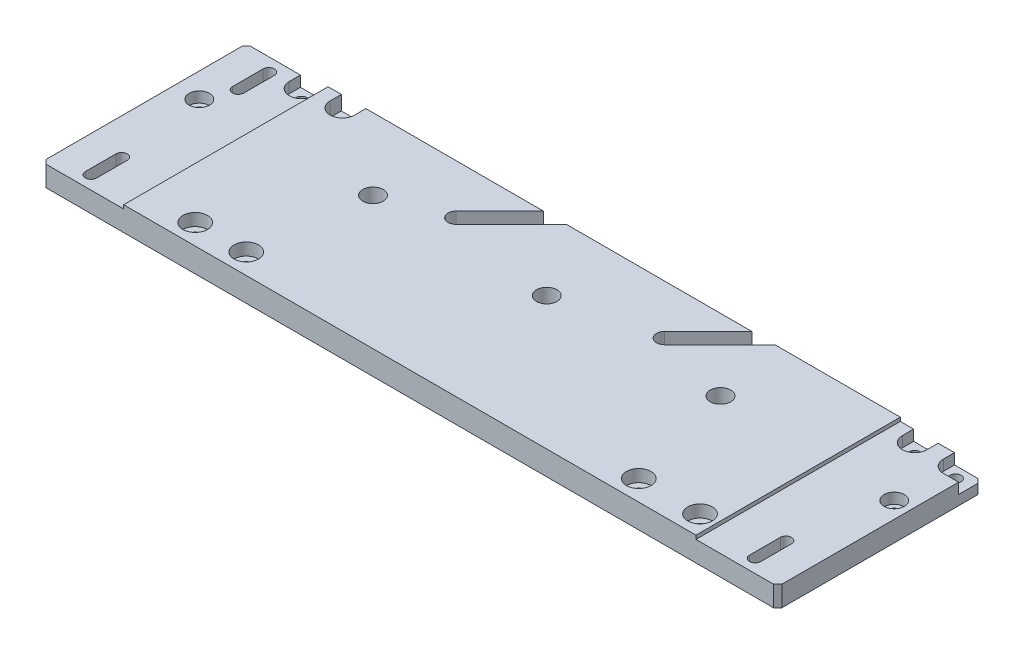
SolidWorks part; units mm, degrees
ref_plane "Front Plane" through (0, 0, 0) normal (0, 0, 1) x (1, 0, 0)
ref_plane "Top Plane" through (0, 0, 0) normal (0, 1, 0) x (1, 0, 0)
ref_plane "Right Plane" through (0, 0, 0) normal (1, 0, 0) x (0, 0, -1)
sketch "Sketch1" plane through (0, 0, 0) normal (0, 1, 0) x (1, 0, 0)
  line L1 (-180, 50) -> (180, 50)
  line L2 (-180, 50) -> (-180, -50)
  line L3 (-180, -50) -> (180, -50)
  line L4 (180, 50) -> (180, -50)
  line L5 (-180, 50) -> (180, -50) construction
  line L6 (-180, -50) -> (180, 50) construction
  point P0 (0, 0)
  dimension "D1" = 360
  dimension "D2" = 100
extrude "Boss-Extrude1" add sketch "Sketch1" along normal blind 10
sketch "Sketch2" plane through (0, 10, 0) normal (0, 1, 0) x (1, 0, 0)
  line L0 (180, 50) -> (-180, 50) construction
  line L1 (-140, -50) -> (140, -50)
  line L2 (-140, -50) -> (-140, 50)
  line L3 (-140, 50) -> (140, 50)
  line L4 (140, -50) -> (140, 50)
  line L5 (-140, -50) -> (140, 50) construction
  line L6 (-140, 50) -> (140, -50) construction
  point P0 (0, 0)
  dimension "D1" = 280
extrude "Boss-Extrude2" add sketch "Sketch2" along normal blind 1.8
sketch "Sketch3" plane through (0, 0, 0) normal (0, -1, 0) x (1, 0, 0)
  line L0 (-32.2377, -40) -> (49967.7623, -40) construction
  line L2 (-180, -50) -> (-180, 50) construction
  line L3 (180, -50) -> (-180, -50) construction
  circle A0 centre (-39, -40) radius 4
  circle A1 centre (63, -40) radius 4
  dimension "D1" = 102
  dimension "D3" = 8
  dimension "D4" = 141
  dimension "D2" = 10
extrude "Cut-Extrude1" cut sketch "Sketch3" against normal through all
sketch "Sketch4" plane through (0, 0, 0) normal (0, -1, 0) x (1, 0, 0)
  line L0 (-56.0102, -57.0102) -> (35299.3289, 35298.3289) construction
  line L1 (53.9844, -49.0156) -> (35409.3234, 35306.3234) construction
  line L3 (180, -50) -> (-180, -50) construction
  line L4 (-64.5, -14.5) -> (35290.8391, -35369.8391) construction
  line L5 (44, -21) -> (35399.3391, -35376.3391) construction
  line L6 (48.8579, -25.8579) -> (77.1421, -54.1421) construction
  line L7 (51.6863, -23.0294) -> (79.9706, -51.3137)
  line L8 (46.0294, -28.6863) -> (74.3137, -56.9706)
  line L9 (-53.1421, -25.8579) -> (-24.8579, -54.1421) construction
  line L10 (-50.3137, -23.0294) -> (-22.0294, -51.3137)
  line L11 (-55.9706, -28.6863) -> (-27.6863, -56.9706)
  arc A0 (51.6863, -23.0294) -> (46.0294, -28.6863) centre (48.8579, -25.8579) ccw
  arc A1 (74.3137, -56.9706) -> (79.9706, -51.3137) centre (77.1421, -54.1421) ccw
  arc A2 (-50.3137, -23.0294) -> (-55.9706, -28.6863) centre (-53.1421, -25.8579) ccw
  arc A3 (-27.6863, -56.9706) -> (-22.0294, -51.3137) centre (-24.8579, -54.1421) ccw
  circle A4 centre (-39, -40) radius 4 construction
  point P14 (63, -40)
  point P20 (-39, -40)
  dimension "D1" = 45
  dimension "D2" = 40
  dimension "D3" = 40
extrude "Cut-Extrude2" cut sketch "Sketch4" against normal blind 39
sketch "Sketch5" plane through (0, 0, 0) normal (0, -1, 0) x (1, 0, 0)
  line L0 (-160, 0) -> (49840, 0) construction
  line L1 (-180, -50) -> (-180, 50) construction
  line L2 (-162.504, 43.5) -> (-162.496, 28.5) construction
  line L3 (-159.754, 43.5015) -> (-159.746, 28.5015)
  line L4 (-165.254, 43.4985) -> (-165.246, 28.4985)
  line L6 (0, 50) -> (0, -49950) construction
  line L7 (-180, 50) -> (180, 50) construction
  line L8 (162.5, 43.5) -> (162.5, 28.5) construction
  line L9 (159.75, 43.5) -> (159.75, 28.5)
  line L10 (165.25, 43.5) -> (165.25, 28.5)
  line L23 (-162.504, -43.5) -> (-162.496, -28.5) construction
  line L24 (-159.754, -43.5015) -> (-159.746, -28.5015)
  line L25 (-165.254, -43.4985) -> (-165.246, -28.4985)
  arc A0 (-159.754, 43.5015) -> (-165.254, 43.4985) centre (-162.504, 43.5) ccw
  arc A1 (-165.246, 28.4985) -> (-159.746, 28.5015) centre (-162.496, 28.5) ccw
  arc A2 (159.75, 43.5) -> (165.25, 43.5) centre (162.5, 43.5) cw
  arc A3 (165.25, 28.5) -> (159.75, 28.5) centre (162.5, 28.5) cw
  arc A12 (-159.754, -43.5015) -> (-165.254, -43.4985) centre (-162.504, -43.5) cw
  arc A13 (-165.246, -28.4985) -> (-159.746, -28.5015) centre (-162.496, -28.5) cw
  point P4 (-180, 0)
  point P7 (-162.5, 36)
  point P18 (0, 50)
  point P19 (162.5, 36)
  point P55 (-162.5, -36)
  dimension "D1" = 5.5
  dimension "D2" = 15
  dimension "D3" = 325
  dimension "D4" = 72
  dimension "D5" = 5.5
  dimension "D6" = 15
extrude "Cut-Extrude3" cut sketch "Sketch5" against normal blind 39
chamfer "Chamfer1" distance 2 angle 45 6 edges at (180, 5, 50) (-180, 5, 50) (-180, 5, -50) (180, 5, -50)
sketch "Sketch6" plane through (0, 11.8, 0) normal (0, 1, 0) x (1, 0, 0)
  line L0 (180, -48) -> (180, 48) construction
  line L1 (-140, -50) -> (140, -50) construction
  circle A0 centre (132, -40) radius 2.75
  circle A1 centre (102, -40) radius 2.75
  circle A2 centre (-90, -40) radius 2.75
  circle A3 centre (-115, -40) radius 2.75
  dimension "D6" = 5.5
  dimension "D1" = 30
  dimension "D2" = 25
  dimension "D3" = 48
  dimension "D4" = 270
  dimension "D5" = 10
extrude "Cut-Extrude4" cut sketch "Sketch6" against normal through all
sketch "Sketch7" plane through (0, 11.8, 0) normal (0, 1, 0) x (1, 0, 0)
  circle A0 centre (-115, -40) radius 6
  circle A1 centre (-90, -40) radius 6
  circle A2 centre (102, -40) radius 6
  circle A3 centre (132, -40) radius 6
  dimension "D1" = 12
extrude "Cut-Extrude5" cut sketch "Sketch7" against normal blind 6
sketch "Sketch8" plane through (0, 11.8, 0) normal (0, 1, 0) x (1, 0, 0)
  line L0 (-180, 48) -> (-180, -48) construction
  line L1 (-34.6569, 50) -> (-140, 50) construction
  circle A0 centre (-147.5, 44.5) radius 2.75
  circle A1 centre (-127.5, 44.5) radius 2.75
  dimension "D1" = 5.5
  dimension "D2" = 20
  dimension "D3" = 32.5
  dimension "D4" = 5.5
extrude "Cut-Extrude6" cut sketch "Sketch8" against normal blind 19
sketch "Sketch9" plane through (0, 11.8, 0) normal (0, 1, 0) x (1, 0, 0)
  circle A0 centre (-147.5, 44.5) radius 6
  circle A1 centre (-127.5, 44.5) radius 6
  dimension "D1" = 12
extrude "Cut-Extrude7" cut sketch "Sketch9" against normal blind 7
sketch "Sketch11" plane through (0, 11.8, 0) normal (0, 1, 0) x (1, 0, 0)
  line L0 (-147.5, 44.5) -> (-147.5, 50044.5) construction
  line L1 (-127.5, 44.5) -> (-127.5, 50044.5) construction
  line L2 (-125.1021, 50) -> (-129.8979, 50) construction
  line L3 (-153.5, 56.0023) -> (-141.5, 56.0023)
  line L4 (-153.5, 56.0023) -> (-153.5, 44.5)
  line L5 (-153.5, 44.5) -> (-141.5, 44.5)
  line L6 (-141.5, 56.0023) -> (-141.5, 44.5)
  line L7 (-153.5, 56.0023) -> (-141.5, 44.5) construction
  line L8 (-153.5, 44.5) -> (-141.5, 56.0023) construction
  line L9 (-133.5, 55.5) -> (-121.5, 55.5)
  line L10 (-133.5, 55.5) -> (-133.5, 44.5)
  line L11 (-133.5, 44.5) -> (-121.5, 44.5)
  line L12 (-121.5, 55.5) -> (-121.5, 44.5)
  line L13 (-133.5, 55.5) -> (-121.5, 44.5) construction
  line L14 (-133.5, 44.5) -> (-121.5, 55.5) construction
  arc A0 (-149.8979, 50) -> (-145.1021, 50) centre (-147.5, 44.5) ccw construction
  arc A1 (-149.8979, 50) -> (-145.1021, 50) centre (-147.5, 44.5) ccw construction
  arc A2 (-129.8979, 50) -> (-125.1021, 50) centre (-127.5, 44.5) ccw construction
  arc A3 (-129.8979, 50) -> (-125.1021, 50) centre (-127.5, 44.5) ccw construction
  point P6 (-147.5, 50.2511)
  point P17 (-127.5, 50)
extrude "Cut-Extrude8" cut sketch "Sketch11" against normal up to surface (7 mm away) up to face at (-147.5, 4.8, -41.75)
sketch "Sketch12" plane through (0, 11.8, 0) normal (0, 1, 0) x (1, 0, 0)
  line L0 (-180, 48) -> (-180, -48) construction
  line L1 (-178, -50) -> (-140, -50) construction
  circle A0 centre (-168, 15) radius 2.75
  dimension "D1" = 5.5
  dimension "D2" = 12
  dimension "D3" = 65
extrude "Cut-Extrude9" cut sketch "Sketch12" against normal through all
pattern_linear "LPattern1" count 5 spacing 85 along (1, 0, 0) of "Cut-Extrude9"
sketch "Sketch13" plane through (0, 11.8, 0) normal (0, 1, 0) x (1, 0, 0)
  circle A0 centre (172, 15) radius 5
  circle A1 centre (87, 15) radius 5
  circle A2 centre (2, 15) radius 5
  circle A3 centre (-83, 15) radius 5
  circle A4 centre (-168, 15) radius 5
  dimension "D1" = 10
extrude "Cut-Extrude10" cut sketch "Sketch13" against normal blind 7
sketch "Sketch14" plane through (0, 0, 0) normal (0, -1, 0) x (1, 0, 0)
  circle A0 centre (152.5, -44.5) radius 2.75
  circle A1 centre (172.5, -44.5) radius 2.75
  dimension "D1" = 5.5
extrude "Cut-Extrude11" cut sketch "Sketch14" against normal blind 10
sketch "Sketch15" plane through (0, 10, 0) normal (0, 1, 0) x (1, 0, 0)
  circle A0 centre (152.5, 44.5) radius 6
  circle A1 centre (172.5, 44.5) radius 6
  arc A2 (-133.5, 44.5) -> (-121.5, 44.5) centre (-127.5, 44.5) ccw construction
extrude "Cut-Extrude12" cut sketch "Sketch15" against normal up to surface (5.2 mm away)
sketch "Sketch16" plane through (0, 10, 0) normal (0, 1, 0) x (1, 0, 0)
  line L0 (152.5, 44.5) -> (50152.5, 44.5) construction
  line L1 (172.5, 44.5) -> (172.5, 50044.5) construction
  line L2 (152.5, 44.5) -> (152.5, 50044.5) construction
  line L3 (154.8979, 50) -> (150.1021, 50) construction
  line L4 (146.5, 55.5) -> (158.5, 55.5)
  line L5 (146.5, 55.5) -> (146.5, 44.5)
  line L6 (146.5, 44.5) -> (158.5, 44.5)
  line L7 (158.5, 55.5) -> (158.5, 44.5)
  line L8 (146.5, 55.5) -> (158.5, 44.5) construction
  line L9 (146.5, 44.5) -> (158.5, 55.5) construction
  line L10 (174.8979, 50) -> (170.1021, 50) construction
  line L11 (178.5, 55.5) -> (166.5, 55.5)
  line L12 (178.5, 55.5) -> (178.5, 44.5)
  line L13 (178.5, 44.5) -> (166.5, 44.5)
  line L14 (166.5, 55.5) -> (166.5, 44.5)
  line L15 (178.5, 55.5) -> (166.5, 44.5) construction
  line L16 (178.5, 44.5) -> (166.5, 55.5) construction
  arc A0 (150.1021, 50) -> (154.8979, 50) centre (152.5, 44.5) ccw construction
  arc A1 (170.1021, 50) -> (174.8979, 50) centre (172.5, 44.5) ccw construction
  point P8 (152.5, 50)
  point P18 (172.5, 50)
extrude "Cut-Extrude13" cut sketch "Sketch16" against normal up to surface (5.2 mm away) up to face at (152.5, 4.8, -41.75)
sketch "Sketch17" plane through (0, 10, 0) normal (0, 1, 0) x (1, 0, 0)
  line L1 (184.5, 50.5) -> (172.5, 50.5)
  line L2 (184.5, 50.5) -> (184.5, 38.5)
  line L3 (184.5, 38.5) -> (172.5, 38.5)
  line L4 (172.5, 50.5) -> (172.5, 38.5)
  line L5 (184.5, 50.5) -> (172.5, 38.5) construction
  line L6 (184.5, 38.5) -> (172.5, 50.5) construction
  arc A0 (166.5, 44.5) -> (178.5, 44.5) centre (172.5, 44.5) ccw construction
  point P0 (178.5, 44.5)
extrude "Cut-Extrude14" cut sketch "Sketch17" against normal up to surface (5.2 mm away) up to face at (172.5, 4.8, -41.75)
